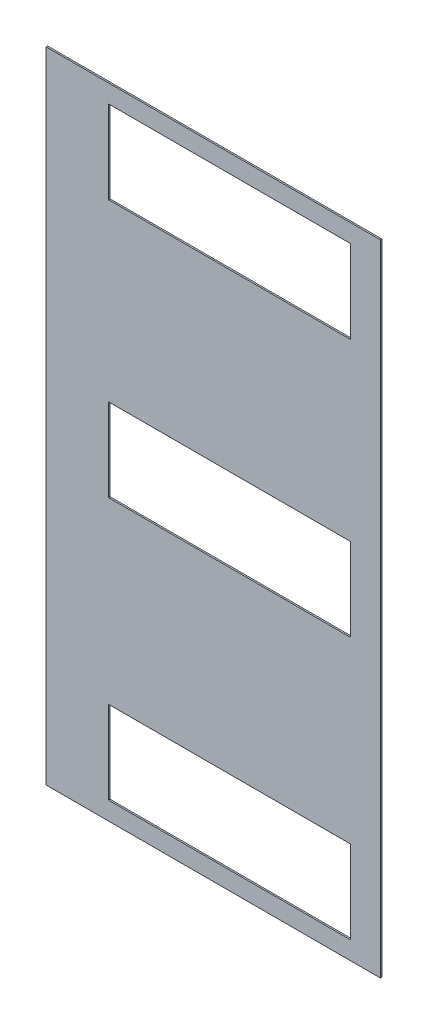
from build123d import *

# Parameters (mm, degrees)
SKETCH1_W           = 1110.611762236
SKETCH1_H           = 2124
SKETCH1_W_2         = 805.022462921
SKETCH1_H_2         = 275.761568038
BOSS_EXTRUDE1_DEPTH = 5


with BuildPart() as part:
    # Sketch1 → Boss-Extrude1 (new body)
    with BuildSketch(Plane.XY):
        with Locations((555.305881118, 1062)):
            Rectangle(SKETCH1_W, SKETCH1_H)
        with Locations((609.562824722, 1925.776054905)):
            Rectangle(SKETCH1_W_2, SKETCH1_H_2, mode=Mode.SUBTRACT)
        with Locations((609.562824722, 1068.55899332)):
            Rectangle(SKETCH1_W_2, SKETCH1_H_2, mode=Mode.SUBTRACT)
        with Locations((609.562824722, 198.131798559)):
            Rectangle(SKETCH1_W_2, SKETCH1_H_2, mode=Mode.SUBTRACT)
    extrude(amount=BOSS_EXTRUDE1_DEPTH)


solid = part.part
